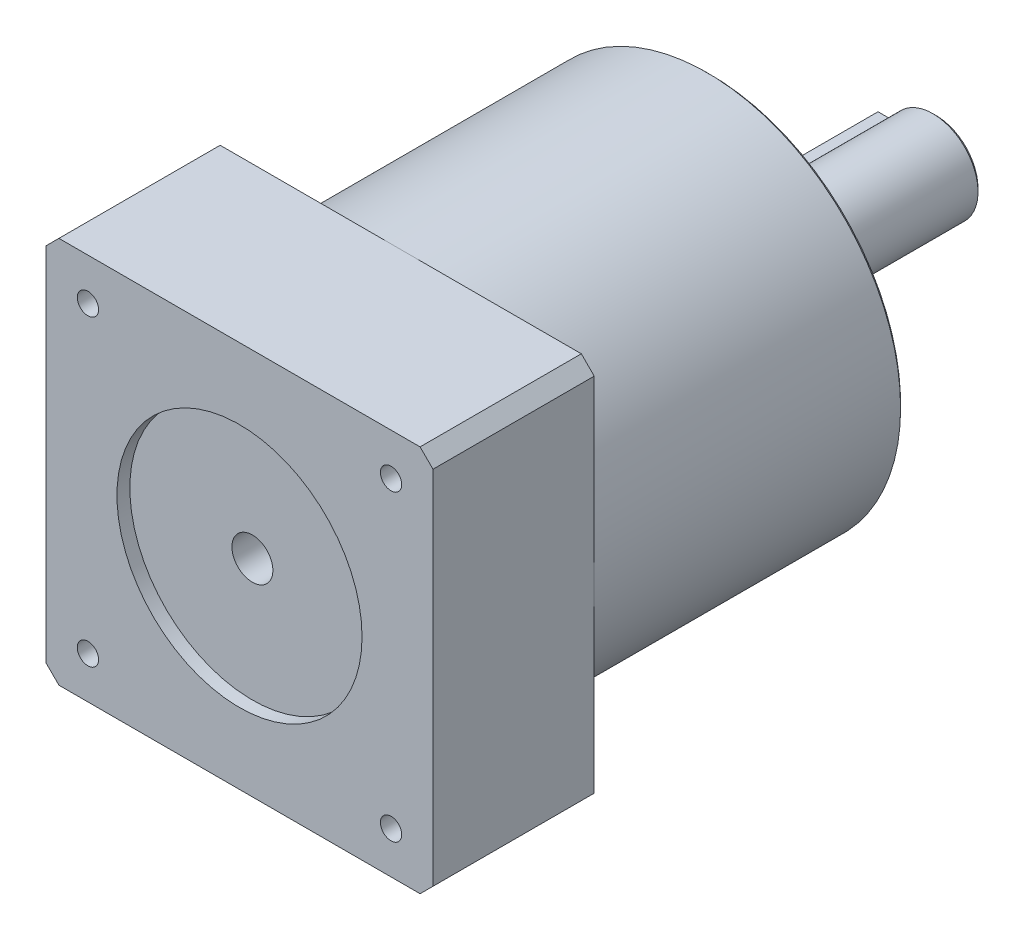
SolidWorks part; units mm, degrees
material "6061"
ref_plane "前视基准面" through (0, 0, 0) normal (0, 0, 1) x (1, 0, 0)
ref_plane "上视基准面" through (0, 0, 0) normal (0, 1, 0) x (1, 0, 0)
ref_plane "右视基准面" through (0, 0, 0) normal (1, 0, 0) x (0, 0, -1)
sketch "草图1" plane through (0, 0, 0) normal (0, 0, 1) x (1, 0, 0)
  line L1 (-30, -30) -> (30, -30)
  line L2 (-30, -30) -> (-30, 30)
  line L3 (-30, 30) -> (30, 30)
  line L4 (30, -30) -> (30, 30)
  line L5 (-30, -30) -> (30, 30) construction
  line L6 (-30, 30) -> (30, -30) construction
  point P0 (0, 0)
  dimension "D1" = 60
  dimension "D2" = 60
extrude "凸台-拉伸1" add sketch "草图1" along normal blind 25
sketch "草图2" plane through (0, 0, 0) normal (0, 0, -1) x (-1, 0, 0)
  circle A0 centre (0, 0) radius 30
  dimension "D1" = 60
extrude "凸台-拉伸2" add sketch "草图2" along normal blind 48
sketch "草图3" plane through (0, 0, -48) normal (0, 0, -1) x (-1, 0, 0)
  circle A0 centre (0, 0) radius 20
  dimension "D1" = 40
extrude "凸台-拉伸3" add sketch "草图3" along normal blind 3
sketch "草图4" plane through (0, 0, -51) normal (0, 0, -1) x (-1, 0, 0)
  circle A0 centre (0, 0) radius 8.5
  dimension "D1" = 17
extrude "凸台-拉伸4" add sketch "草图4" along normal blind 2
sketch "草图5" plane through (0, 0, -53) normal (0, 0, -1) x (-1, 0, 0)
  circle A0 centre (0, 0) radius 7
  dimension "D1" = 14
extrude "凸台-拉伸5" add sketch "草图5" along normal blind 30
sketch "草图7" plane through (0, 0, 25) normal (0, 0, 1) x (1, 0, 0)
  circle A0 centre (0, 0) radius 3.175
  dimension "D1" = 6.35
extrude "切除-拉伸1" cut sketch "草图7" against normal blind 21
sketch "草图8" plane through (0, 0, 25) normal (0, 0, 1) x (1, 0, 0)
  circle A0 centre (0, 0) radius 19
  dimension "D1" = 38
extrude "切除-拉伸2" cut sketch "草图8" against normal blind 2
hole_wizard "M4 螺纹孔1" positions "草图11" profile "草图10" tap size "M4" standard "GB"
sketch "草图11" plane through (0, 0, 25) normal (0, 0, 1) x (1, 0, 0)
  point P0 (23.5, 23.5)
  dimension "D1" = 23.5
  dimension "D2" = 23.5
sketch "草图10" plane through (23.5, 23.5, 25) normal (1, 0, 0) x (0, -1, 0)
  line L0 (0, 0) -> (0, 12.4914)
  line L1 (0, 12.4914) -> (1.65, 11.5)
  line L2 (1.65, 11.5) -> (1.65, 0)
  line L5 (1.65, 0) -> (0, 0)
  line L10 (0, 12.4914) -> (-1.65, 11.5) construction
  line L11 (0, -6.35) -> (0, 107.95) construction
  dimension "螺纹孔钻头直径" = 3.3
  dimension "螺纹孔钻头深度" = 11.5
  dimension "导头角度" = 118
cosmetic thread "孔螺蚊线1" parameters "D1"=8, "D2"=4
hole_wizard "M5 螺纹孔1" positions "草图16" profile "草图15" tap size "M5" standard "GB"
sketch "草图16" plane through (0, 0, -48) normal (0, 0, -1) x (-1, 0, 0)
  line L0 (0, 0) -> (36.7696, 36.7696) construction
  line L2 (0, 0) -> (53.2864, 0) construction
  circle A1 centre (0, 0) radius 26 construction
  point P0 (18.3848, 18.3848)
  dimension "D1" = 52
  dimension "D2" = 45
sketch "草图15" plane through (-18.3848, 18.3848, -48) normal (1, 0, 0) x (0, 1, 0)
  line L0 (0, 0) -> (0, 13.2618)
  line L1 (0, 13.2618) -> (2.1, 12)
  line L2 (2.1, 12) -> (2.1, 0)
  line L5 (2.1, 0) -> (0, 0)
  line L10 (0, 13.2618) -> (-2.1, 12) construction
  line L11 (0, -6.35) -> (0, 107.95) construction
  dimension "螺纹孔钻头直径" = 4.2
  dimension "螺纹孔钻头深度" = 12
  dimension "导头角度" = 118
cosmetic thread "孔螺蚊线2" parameters "D1"=8, "D2"=5
pattern_circular "阵列(圆周)1" count 4 over 360 about axis through (0, 0, 0) along (0, 0, 1) of "M4 螺纹孔1", "M5 螺纹孔1"
chamfer "倒角1" distance 2 angle 45 4 edges at (-30, 30, 12.5) (-30, -30, 12.5) (30, -30, 12.5) (30, 30, 12.5)
sketch "草图17" plane through (0, 0, -83) normal (0, 0, -1) x (-1, 0, 0)
  line L1 (5, -2.5) -> (9, -2.5)
  line L2 (5, -2.5) -> (5, 2.5)
  line L3 (5, 2.5) -> (9, 2.5)
  line L4 (9, -2.5) -> (9, 2.5)
  line L5 (5, -2.5) -> (9, 2.5) construction
  line L6 (5, 2.5) -> (9, -2.5) construction
  circle A0 centre (0, 0) radius 7 construction
  circle A1 centre (0, 0) radius 7 construction
  point P0 (7, 0)
  dimension "D1" = 5
  dimension "D2" = 9
extrude "凸台-拉伸6" add sketch "草图17" against normal blind 27.5
chamfer "倒角2" distance 0.5 angle 45 2 edges at (7, 0, -83) (-30, 0, -48)
